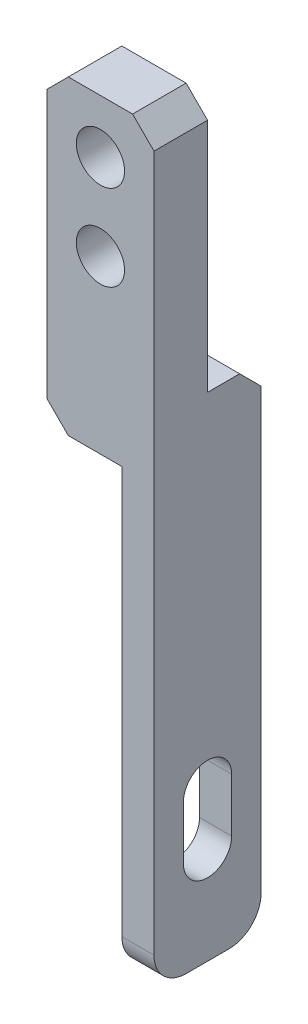
from build123d import *

# Parameters (mm, degrees)
SKETCH1_W            = 10
SKETCH1_H            = 70
BOSS_EXTRUDE1_DEPTH  = 5
SKETCH2_W            = 7
SKETCH2_H            = 41
CUT_EXTRUDE1_DEPTH   = 37.742346142
SKETCH3_W            = 5
SKETCH3_H            = 24
CUT_EXTRUDE2_DEPTH   = 37.742346142
CUT_EXTRUDE3_DEPTH   = 37.742346142
FILLET1_R            = 3
M4_CLEARANCE_HOLE1_D = 4.5
CHAMFER1_SIZE        = 2


with BuildPart() as part:
    # Sketch1 → Boss-Extrude1 (new, symmetric)
    with BuildSketch(Plane.XY):
        Rectangle(SKETCH1_W, SKETCH1_H)
    extrude(amount=BOSS_EXTRUDE1_DEPTH, both=True)

    # Sketch2 → Cut-Extrude1 (cut, through all)
    with BuildSketch(Plane.XY.offset(5)):
        with Locations((-1.5, -14.5)):
            Rectangle(SKETCH2_W, SKETCH2_H)
    extrude(amount=-CUT_EXTRUDE1_DEPTH, mode=Mode.SUBTRACT)

    # Sketch3 → Cut-Extrude2 (cut, through all)
    with BuildSketch(Plane(origin=(5, 0, 0), x_dir=(0, 0, -1), z_dir=(1, 0, 0))):
        with Locations((2.5, 23)):
            Rectangle(SKETCH3_W, SKETCH3_H)
    extrude(amount=-CUT_EXTRUDE2_DEPTH, mode=Mode.SUBTRACT)

    # Sketch4 → Cut-Extrude3 (cut, through all)
    with BuildSketch(Plane.ZY.offset(5)):
        with BuildLine():
            Line((2.25, -21), (2.25, -26))
            ThreePointArc((2.25, -26), (0, -28.25), (-2.25, -26))
            Line((-2.25, -26), (-2.25, -21))
            ThreePointArc((-2.25, -21), (0, -18.75), (2.25, -21))
        make_face()
    extrude(amount=-CUT_EXTRUDE3_DEPTH, mode=Mode.SUBTRACT)

    # Fillet1
    fillet1_edges = [part.edges().sort_by_distance(p)[0] for p in [
        (3.5, -35, -5),
        (3.5, -35, 5),
    ]]
    fillet(fillet1_edges, radius=FILLET1_R)

    # M4 Clearance Hole1 (through all)
    with Locations(Plane.XY.offset(5)):
        with Locations((0, 30), (0, 22)):
            Hole(M4_CLEARANCE_HOLE1_D / 2)

    # Chamfer1
    chamfer1_edges = [part.edges().sort_by_distance(p)[0] for p in [
        (-5, 6, 0),
        (0, 11, -5),
        (-5, 35, 2.5),
        (5, 35, 2.5),
    ]]
    chamfer(chamfer1_edges, length=CHAMFER1_SIZE)


solid = part.part
